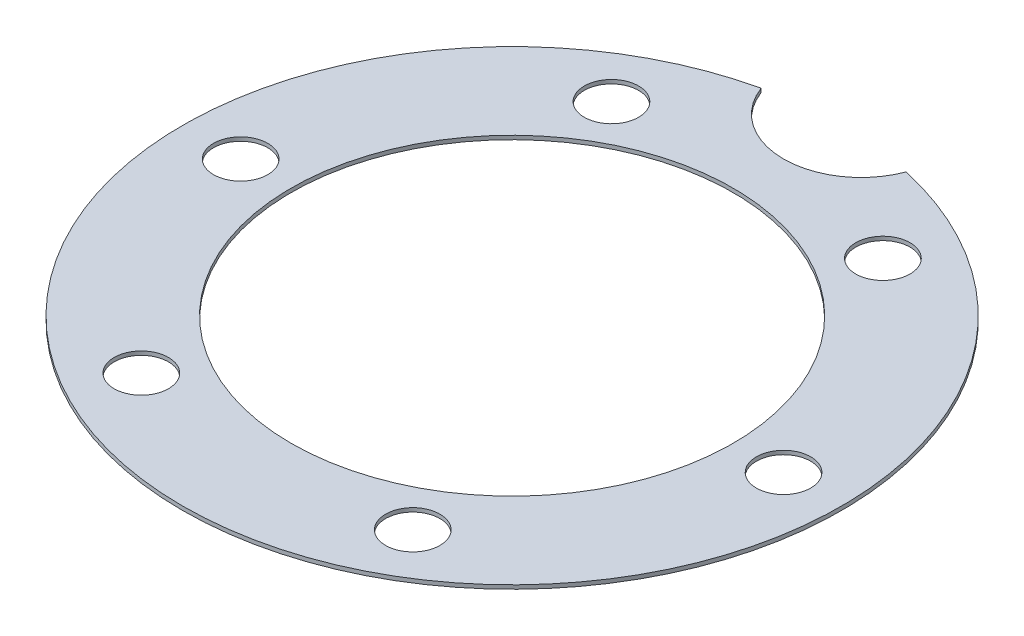
SolidWorks part; units mm, degrees
ref_plane "Front Plane" through (0, 0, 0) normal (0, 0, 1) x (1, 0, 0)
ref_plane "Top Plane" through (0, 0, 0) normal (0, 1, 0) x (1, 0, 0)
ref_plane "Right Plane" through (0, 0, 0) normal (1, 0, 0) x (0, 0, -1)
sketch "Sketch1" plane through (0, 0, 0) normal (0, 1, 0) x (1, 0, 0)
  line L0 (-35, 60.6218) -> (0, 0) construction
  line L1 (0, 0) -> (0, 90) construction
  arc A0 (-18.7036, 82.9167) -> (18.7036, 82.9167) centre (0, 0) ccw
  arc A1 (-18.7036, 82.9167) -> (18.7036, 82.9167) centre (0, 90) ccw
  circle A2 centre (0, 0) radius 70 construction
  circle A3 centre (-35, 60.6218) radius 7
  circle A4 centre (35, 60.6218) radius 7
  circle A5 centre (70, 0) radius 7
  circle A6 centre (35, -60.6218) radius 7
  circle A7 centre (-35, -60.6218) radius 7
  circle A8 centre (-70, 0) radius 7
  circle A9 centre (0, 0) radius 57
  point P20 (0, 0)
  dimension "D1" = 170
  dimension "D2" = 90
  dimension "D3" = 40
  dimension "D4" = 140
  dimension "D5" = 14
  dimension "D8" = 114
  dimension "D6" = 30
  dimension "D7" = 6
extrude "Boss-Extrude1" add sketch "Sketch1" along normal blind 1
